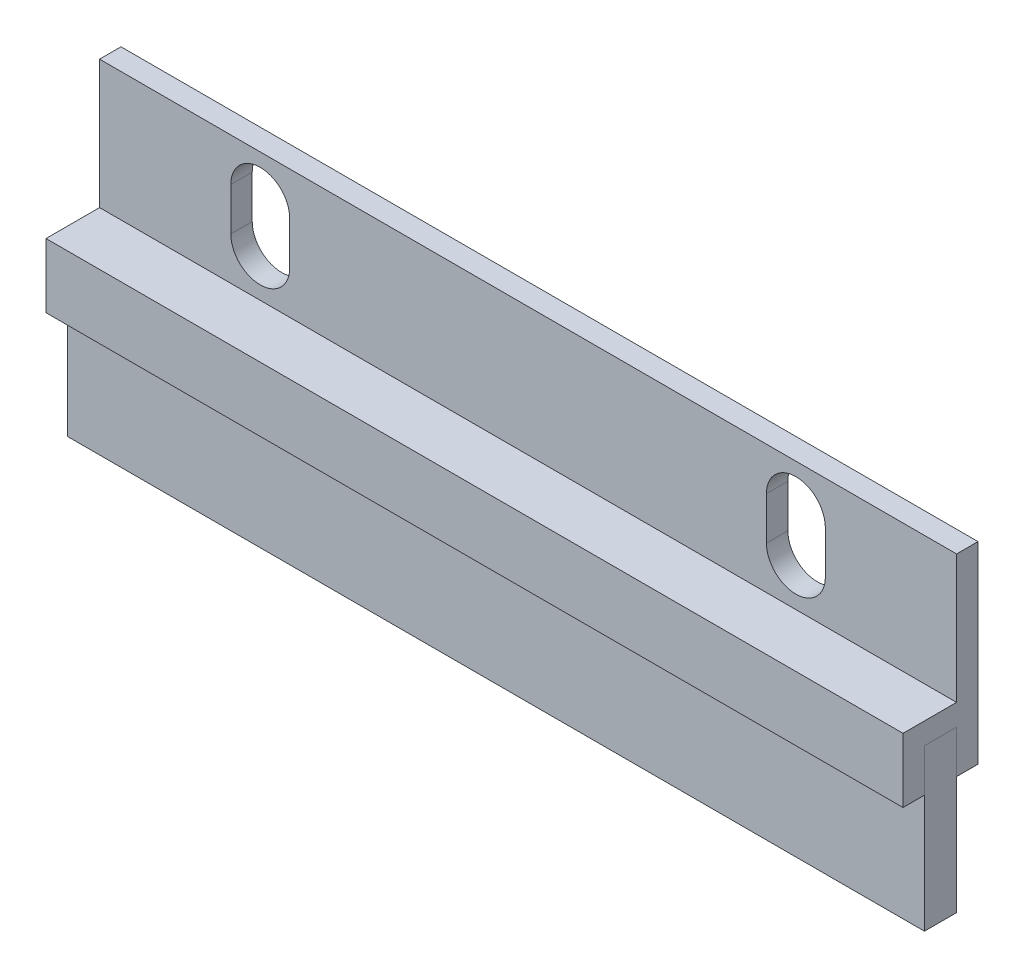
SolidWorks part; units mm, degrees
ref_plane "前视基准面" through (0, 0, 0) normal (0, 0, 1) x (1, 0, 0)
ref_plane "上视基准面" through (0, 0, 0) normal (0, 1, 0) x (1, 0, 0)
ref_plane "右视基准面" through (0, 0, 0) normal (1, 0, 0) x (0, 0, -1)
sketch "草图1" plane through (0, 0, 0) normal (0, 0, 1) x (1, 0, 0)
  line L1 (-40, 18) -> (40, 18)
  line L2 (-40, 18) -> (-40, 0)
  line L3 (-40, 0) -> (40, 0)
  line L4 (40, 18) -> (40, 0)
  dimension "D1" = 18
  dimension "D2" = 80
extrude "凸台-拉伸1" add sketch "草图1" along normal blind 2
sketch "草图2" plane through (0, 0, 2) normal (0, 0, 1) x (1, 0, 0)
  line L0 (-40, 18) -> (-40, 0) construction
  line L1 (-40, 6) -> (40, 6)
  line L2 (-40, 6) -> (-40, 4)
  line L3 (-40, 4) -> (40, 4)
  line L4 (40, 6) -> (40, 4)
  line L5 (40, 0) -> (40, 18) construction
  line L6 (-40, 0) -> (40, 0) construction
  dimension "D1" = 4
  dimension "D2" = 2
extrude "凸台-拉伸2" add sketch "草图2" along normal blind 3
sketch "草图3" plane through (0, 6, 0) normal (0, 1, 0) x (1, 0, 0)
  line L0 (40, -5) -> (40, -2) construction
  line L1 (-40, -5) -> (40, -5)
  line L2 (-40, -5) -> (-40, -7)
  line L3 (-40, -7) -> (40, -7)
  line L4 (40, -5) -> (40, -7)
  dimension "D1" = 2
extrude "凸台-拉伸3" add sketch "草图3" against normal up to surface (6 mm away) up to face at (0, 0, 1)
sketch "草图5" plane through (0, 4, 0) normal (0, -1, 0) x (1, 0, 0)
  line L4 (-40, 2) -> (40, 2)
  line L5 (40, 2) -> (40, 5)
  line L6 (40, 5) -> (-40, 5)
  line L7 (-40, 5) -> (-40, 2)
  line L8 (-40, 2) -> (40, 2)
  line L9 (40, 2) -> (40, 5)
  line L10 (40, 5) -> (-40, 5)
  line L11 (-40, 5) -> (-40, 2)
  dimension "D1" = 0
extrude "凸台-拉伸5" add sketch "草图5" along normal blind 15 separate body
sketch "草图6" plane through (0, 0, 2) normal (0, 0, 1) x (1, 0, 0)
  line L0 (-25, 14) -> (-25, 10) construction
  line L1 (-22.25, 14) -> (-22.25, 10)
  line L2 (-27.75, 14) -> (-27.75, 10)
  line L3 (40, 18) -> (-40, 18) construction
  line L4 (-40, 18) -> (-40, 6) construction
  arc A0 (-22.25, 14) -> (-27.75, 14) centre (-25, 14) ccw
  arc A1 (-27.75, 10) -> (-22.25, 10) centre (-25, 10) ccw
  point P2 (-25, 12)
  dimension "D1" = 2.75
  dimension "D3" = 4
  dimension "D4" = 15
  dimension "D2" = 4
extrude "切除-拉伸1" cut sketch "草图6" against normal blind 5
ref_plane "基准面1" through (0, 0, 0) normal (-1, 0, 0) x (0, 0, 1)
mirror "镜向1" about plane through (0, 0, 0) normal (-1, 0, 0) of "切除-拉伸1"
